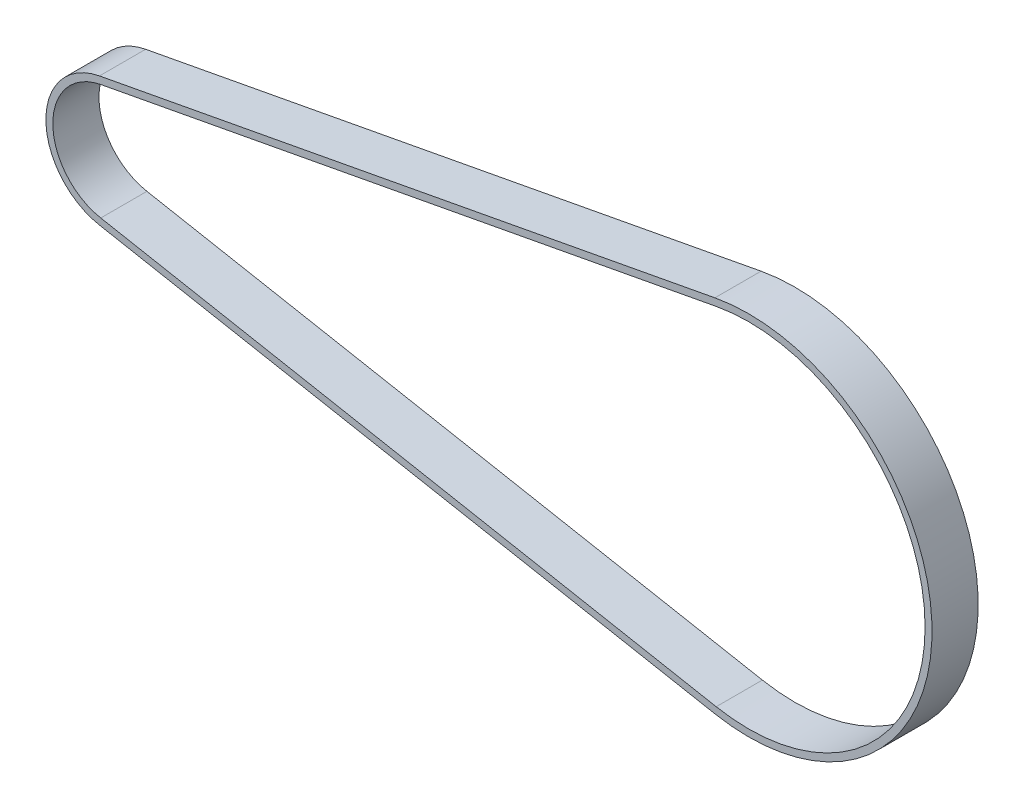
SolidWorks part; units mm, degrees
ref_plane "Front Plane" through (0, 0, 0) normal (0, 0, 1) x (1, 0, 0)
ref_plane "Top Plane" through (0, 0, 0) normal (0, 1, 0) x (1, 0, 0)
ref_plane "Right Plane" through (0, 0, 0) normal (1, 0, 0) x (0, 0, -1)
sketch "Sketch1" plane through (0, 0, 0) normal (0, 0, 1) x (1, 0, 0)
  line L0 (-0.9401, 5.0075) -> (52.3807, 15.0176)
  line L1 (-0.9401, -5.0075) -> (52.3807, -15.0176)
  line L2 (-1.0508, -5.5972) -> (52.27, -15.6073)
  line L3 (-1.0508, 5.5972) -> (52.27, 15.6073)
  arc A0 (-0.9401, 5.0075) -> (-0.9401, -5.0075) centre (0, 0) ccw
  arc A1 (52.3807, -15.0176) -> (52.3807, 15.0176) centre (55.2, 0) ccw
  arc A2 (-1.0508, 5.5972) -> (-1.0508, -5.5972) centre (0, 0) ccw
  arc A3 (52.27, -15.6073) -> (52.27, 15.6073) centre (55.2, 0) ccw
  dimension "D1" = 55.2
  dimension "D2" = 10.19
  dimension "D3" = 30.56
  dimension "D4" = 0.6
extrude "Boss-Extrude1" add sketch "Sketch1" along normal blind 4
